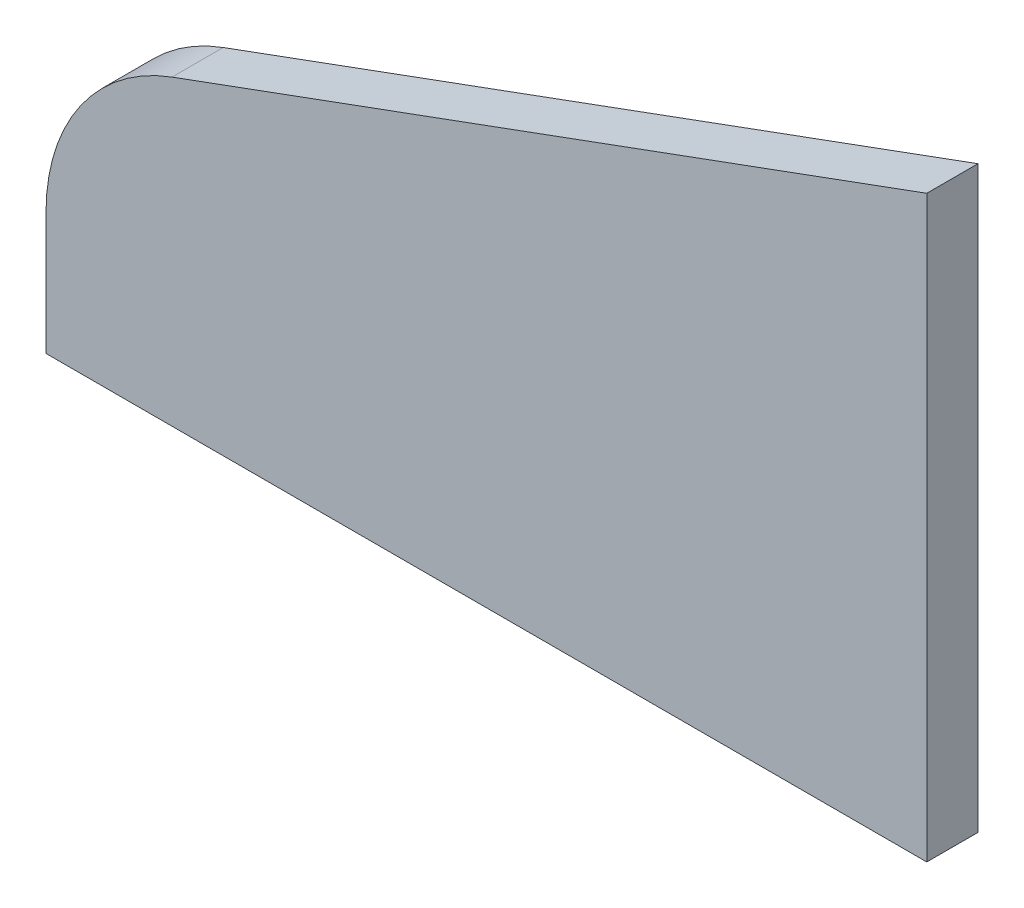
SolidWorks part; units mm, degrees
ref_plane "前视基准面" through (0, 0, 0) normal (0, 0, 1) x (1, 0, 0)
ref_plane "上视基准面" through (0, 0, 0) normal (0, 1, 0) x (1, 0, 0)
ref_plane "右视基准面" through (0, 0, 0) normal (1, 0, 0) x (0, 0, -1)
sketch "草图1" plane through (0, 0, 0) normal (0, 0, 1) x (-1, 0, 0)
  line L0 (-176.4778, -283.4248) -> (-58.6279, -240.2132)
  line L4 (-176.4778, -283.4248) -> (-176.4778, -193)
  line L14 (-38.9556, -212.0469) -> (-38.9556, -193)
  line L15 (-38.9556, -193) -> (-176.4778, -193)
  arc A3 (-58.6279, -240.2132) -> (-38.9556, -212.0469) centre (-68.9556, -212.0469) ccw
extrude "凸台-拉伸1" add sketch "草图1" along normal blind 8
